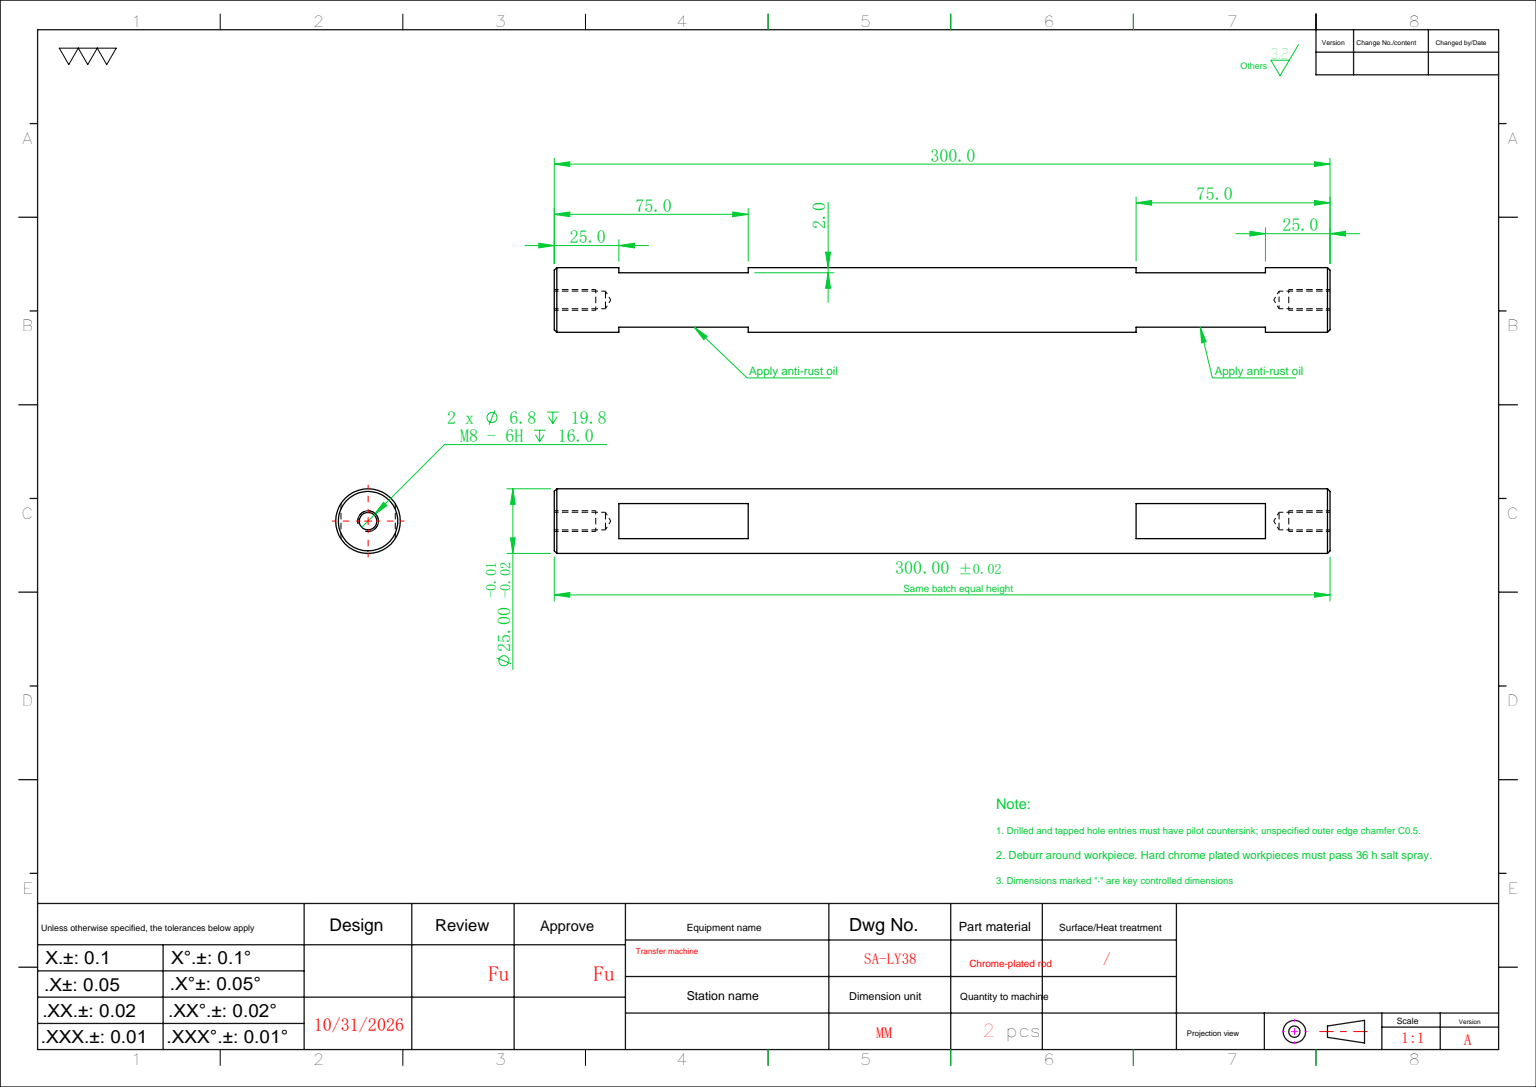
from build123d import *

# Parameters (mm, degrees)
SKETCH_1_R          = 12.5
EXTRUDE_1_DEPTH     = 150
SKETCH_2_W          = 50
SKETCH_2_H          = 2
CUT_EXTRUDE_1_DEPTH = 100
CHAMFER_1_SIZE      = 1


with BuildPart() as part:
    # 草图1 → 凸台-拉伸1 (new, symmetric)
    with BuildSketch(Plane.XY):
        Circle(SKETCH_1_R)
    extrude(amount=EXTRUDE_1_DEPTH, both=True)

    # 草图2 → 切除-拉伸1 (cut, symmetric)
    with BuildSketch(Plane(origin=(0, 0, 0), x_dir=(0, 0, -1), z_dir=(1, 0, 0))):
        with Locations((-100, 11.5)):
            Rectangle(SKETCH_2_W, SKETCH_2_H)
        with Locations((-100, -11.5)):
            Rectangle(SKETCH_2_W, SKETCH_2_H)
        with Locations((100, -11.5)):
            Rectangle(SKETCH_2_W, SKETCH_2_H)
        with Locations((100, 11.5)):
            Rectangle(SKETCH_2_W, SKETCH_2_H)
    extrude(amount=CUT_EXTRUDE_1_DEPTH, both=True, mode=Mode.SUBTRACT)

    # 倒角1
    chamfer_1_edges = [part.edges().sort_by_distance(p)[0] for p in [
        (-12.5, 0, -150),
        (-12.5, 0, 150),
    ]]
    chamfer(chamfer_1_edges, length=CHAMFER_1_SIZE)

    # 草图4 → M8 螺纹孔1 (revolve, cut)
    with BuildSketch(Plane(origin=(0, 0, -150), x_dir=(0, 1, 0), z_dir=(1, 0, 0))):
        Polygon((0, 0), (0, 21.792926105), (3.4, 19.75), (3.4, 0), align=None)
    hole_wizard_m8_1 = revolve(axis=Axis((0, 0, -156.35), (0, 0, 1)), mode=Mode.SUBTRACT)

    # 镜向1: M8 螺纹孔1 across plane
    add(hole_wizard_m8_1.mirror(Plane.XY), mode=Mode.SUBTRACT)


solid = part.part
